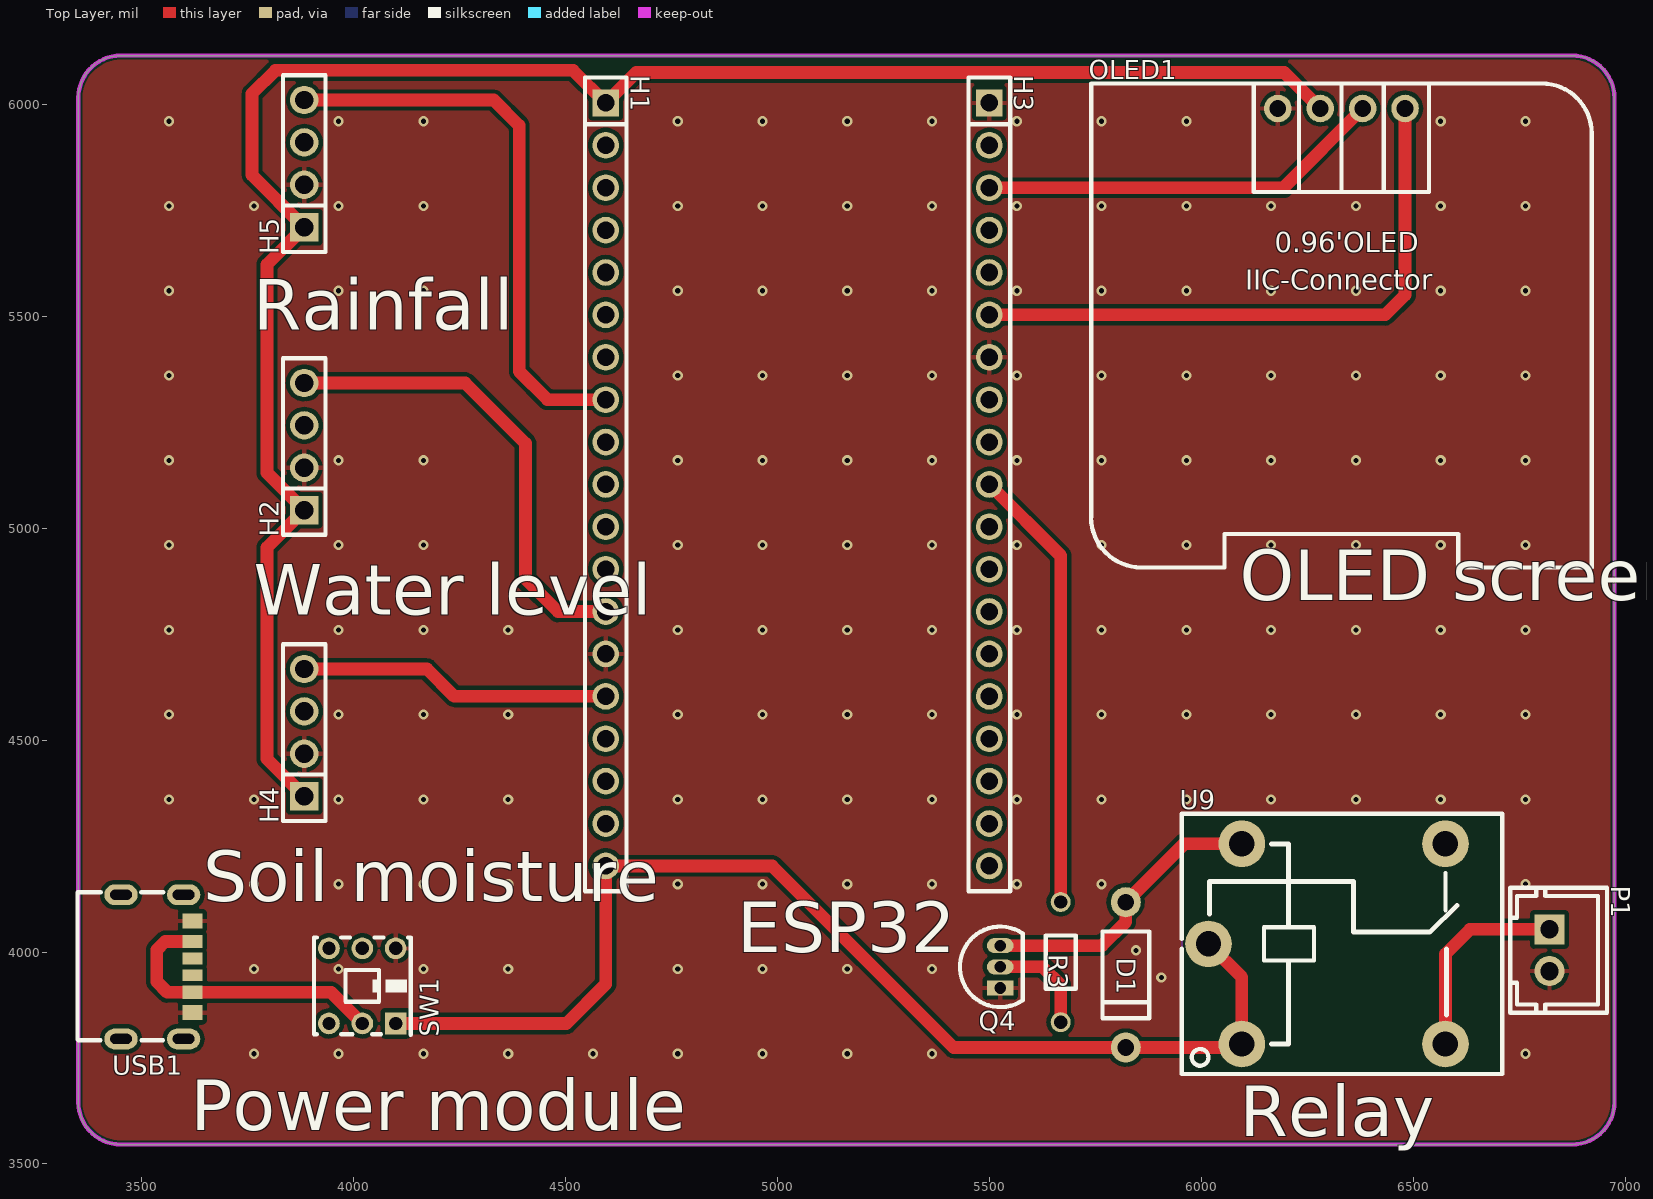
[diagram p0: Top Layer view]
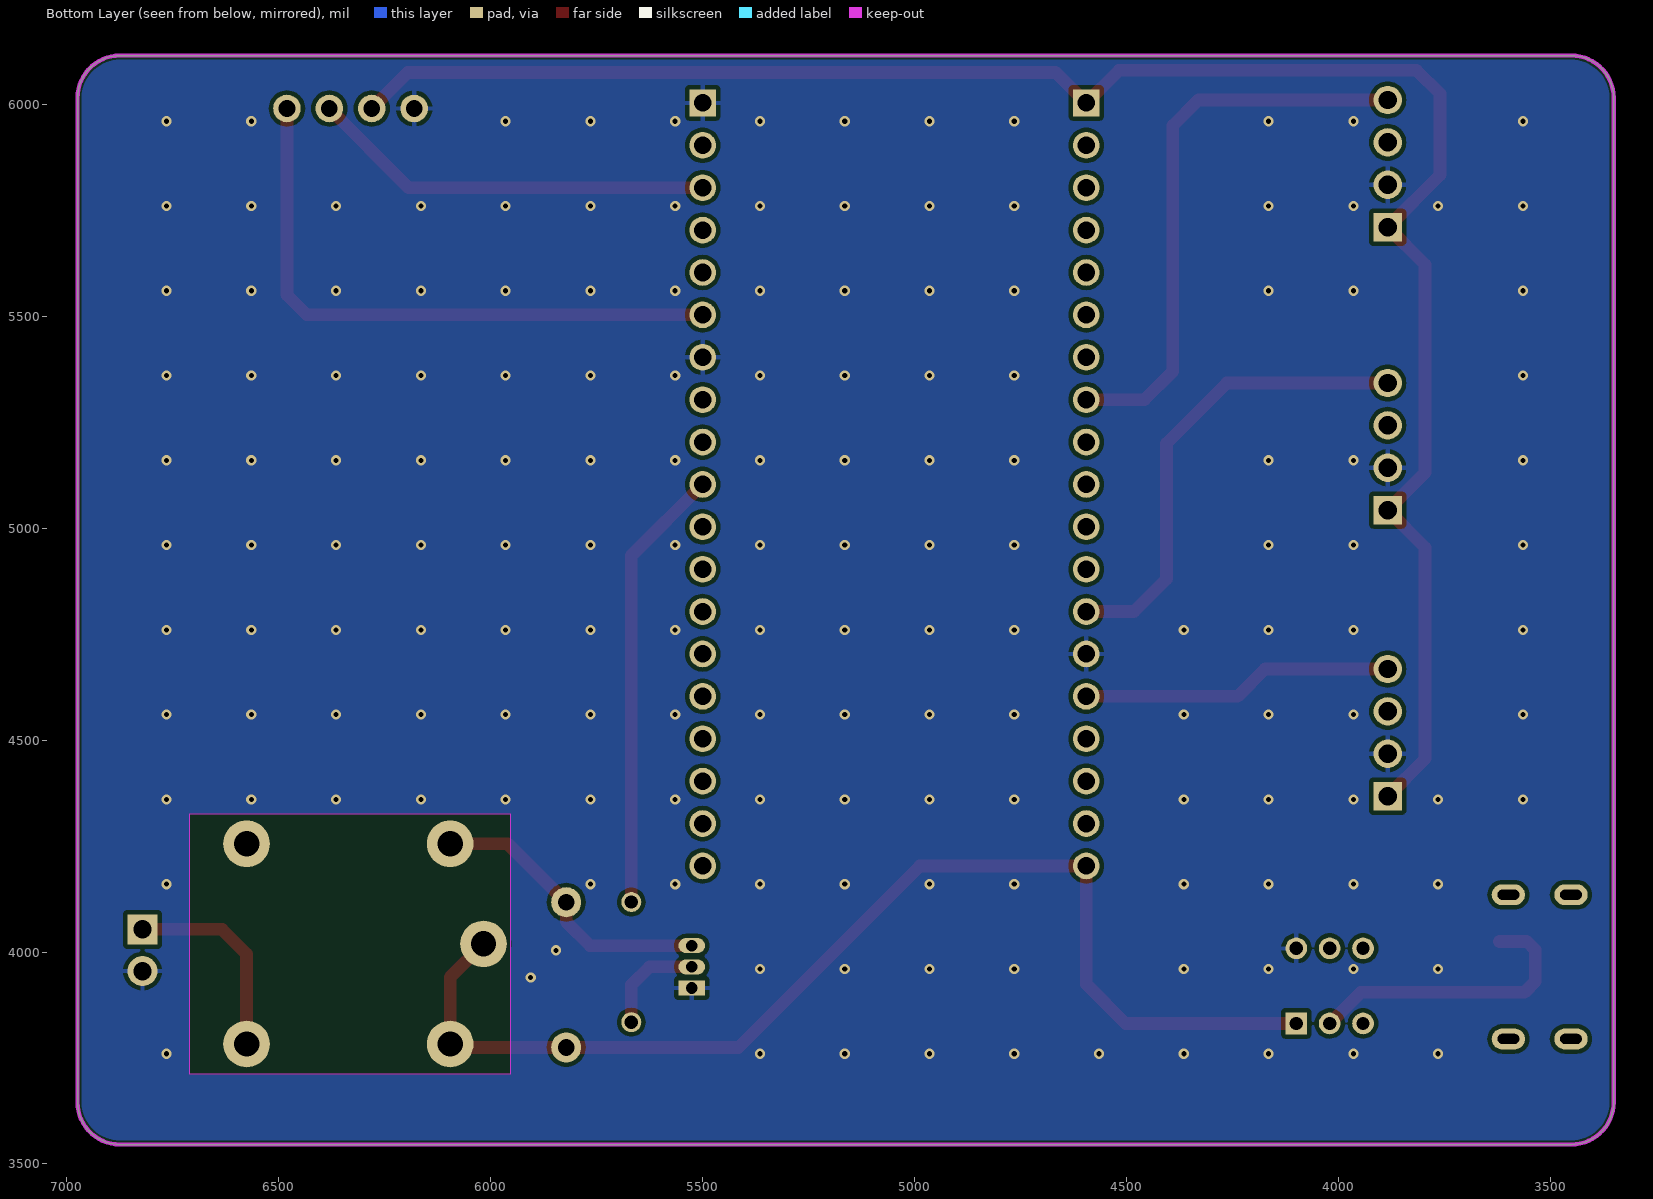
[diagram p1: Bottom Layer view, seen from below]
# Altium PCB MISC89058.pcbdoc
Units mil, origin at the board's own origin, x right, y up, seen from the top; angles counter-clockwise.
Board outline 3624.13 x 2569.13 mil, 2 copper layers (Top Layer, Bottom Layer), stack 62.206 mil thick; 13 components, 40 nets, 84 pads, 158 vias.

## Layer stack, top to bottom
Top Solder Mask Layer: solder mask 0.394, Dk 3.3
Top Layer: signal copper 1.379
Dielectric1: surface 59.449, FR4, Dk 4.5
Bottom Layer: signal copper 1.378
Bottom Solder Mask Layer: solder mask 0.394, Dk 3.3

## Board outline
3450,6115 ccw(c3450,6015) 3350,6015 3350,3645.87 ccw(c3450,3645.87) 3450,3545.87 6874.13,3545.87 ccw(c6874.13,3645.87) 6974.13,3645.87 6974.13,6015 ccw(c6874.13,6015) 6874.13,6115

## Design rules (kind name [scope] priority, off if disabled: settings)
BoardOutlineClearance copperThickness2oz_1 [All] p2 off: genericclearance=7.99 ignorepadtopadclearanceinfootprint=FALSE except(0: Arc-SplitContinuation Track-SplitContinuation SMDPad-SplitContinuation THPad-SplitContinuation Via-SplitContinuation Fill-SplitContinuation Region-SplitContinuation Poly-SplitContinuation Text-SplitContinuation Hole-SplitContinuation; 5.98: Arc-CutoutEdge Track-CutoutEdge SMDPad-CutoutEdge THPad-CutoutEdge Via-CutoutEdge Text-CutoutEdge; 6.9: Hole-OutlineEdge Hole-CutoutEdge; 10: Poly-OutlineEdge Poly-CutoutEdge; 11.81: Arc-OutlineEdge Track-OutlineEdge SMDPad-OutlineEdge THPad-OutlineEdge Via-OutlineEdge Fill-OutlineEdge Region-OutlineEdge Text-OutlineEdge Fill-CutoutEdge Region-CutoutEdge)
BoardOutlineClearance Plane_innerPlane_1 [All] p4 off: genericclearance=4.02 ignorepadtopadclearanceinfootprint=FALSE except(0: Arc-SplitContinuation Track-SplitContinuation SMDPad-SplitContinuation THPad-SplitContinuation Via-SplitContinuation Fill-SplitContinuation Region-SplitContinuation Poly-SplitContinuation Text-SplitContinuation Hole-SplitContinuation; 5.98: Arc-CutoutEdge Track-CutoutEdge SMDPad-CutoutEdge THPad-CutoutEdge Via-CutoutEdge Text-CutoutEdge; 6.9: Hole-OutlineEdge Hole-CutoutEdge; 10: Poly-OutlineEdge Poly-CutoutEdge; 11.81: Arc-OutlineEdge Track-OutlineEdge SMDPad-OutlineEdge THPad-OutlineEdge Via-OutlineEdge Fill-OutlineEdge Region-OutlineEdge Text-OutlineEdge Fill-CutoutEdge Region-CutoutEdge)
BoardOutlineClearance Copper_copperRegion_1 [All] p6 off: genericclearance=4.02 ignorepadtopadclearanceinfootprint=FALSE except(0: Arc-SplitContinuation Track-SplitContinuation SMDPad-SplitContinuation THPad-SplitContinuation Via-SplitContinuation Fill-SplitContinuation Region-SplitContinuation Poly-SplitContinuation Text-SplitContinuation Hole-SplitContinuation; 5.98: Arc-CutoutEdge Track-CutoutEdge SMDPad-CutoutEdge THPad-CutoutEdge Via-CutoutEdge Text-CutoutEdge; 6.9: Hole-OutlineEdge Hole-CutoutEdge; 10: Poly-OutlineEdge Poly-CutoutEdge; 11.81: Arc-OutlineEdge Track-OutlineEdge SMDPad-OutlineEdge THPad-OutlineEdge Via-OutlineEdge Fill-OutlineEdge Region-OutlineEdge Text-OutlineEdge Fill-CutoutEdge Region-CutoutEdge)
BoardOutlineClearance copperThickness1oz_1 [All] p8: genericclearance=4.02 ignorepadtopadclearanceinfootprint=FALSE except(0: Arc-SplitContinuation Track-SplitContinuation SMDPad-SplitContinuation THPad-SplitContinuation Via-SplitContinuation Fill-SplitContinuation Region-SplitContinuation Poly-SplitContinuation Text-SplitContinuation Hole-SplitContinuation; 5.98: Arc-CutoutEdge Track-CutoutEdge SMDPad-CutoutEdge THPad-CutoutEdge Via-CutoutEdge Text-CutoutEdge; 6.9: Hole-OutlineEdge Hole-CutoutEdge; 10: Poly-OutlineEdge Poly-CutoutEdge; 11.81: Arc-OutlineEdge Track-OutlineEdge SMDPad-OutlineEdge THPad-OutlineEdge Via-OutlineEdge Fill-OutlineEdge Region-OutlineEdge Text-OutlineEdge Fill-CutoutEdge Region-CutoutEdge)
Clearance copperThickness2oz [All] p1 off: gap=7.99 ignorepadtopadclearanceinfootprint=FALSE except(5.98: SMDPad-Track SMDPad-SMDPad THPad-Track SMDPad-THPad THPad-THPad Track-Via SMDPad-Via THPad-Via Via-Via Fill-SMDPad Region-SMDPad Fill-THPad Region-THPad Fill-Via Region-Via Fill-Fill Fill-Region Region-Region Arc-Track Arc-SMDPad Arc-THPad Arc-Via Fill-Arc Region-Arc Arc-Arc Text-Track SMDPad-Text Text-THPad Text-Via Fill-Text Region-Text Arc-Text Text-Text; 6.9: Hole-Track Hole-SMDPad Hole-THPad Hole-Via Fill-Hole Region-Hole Hole-Arc Hole-Text; 10: Poly-Track Poly-SMDPad Poly-THPad Poly-Via Poly-Fill Poly-Region Poly-Poly Poly-Arc Poly-Text Poly-Hole; 11.81: Fill-Track Region-Track)
Clearance Plane_innerPlane [All] p3 off: gap=4.02 ignorepadtopadclearanceinfootprint=FALSE except(5.98: SMDPad-Track SMDPad-SMDPad THPad-Track SMDPad-THPad THPad-THPad Track-Via SMDPad-Via THPad-Via Via-Via Fill-SMDPad Region-SMDPad Fill-THPad Region-THPad Fill-Via Region-Via Fill-Fill Fill-Region Region-Region Arc-Track Arc-SMDPad Arc-THPad Arc-Via Fill-Arc Region-Arc Arc-Arc Text-Track SMDPad-Text Text-THPad Text-Via Fill-Text Region-Text Arc-Text Text-Text; 6.9: Hole-Track Hole-SMDPad Hole-THPad Hole-Via Fill-Hole Region-Hole Hole-Arc Hole-Text; 10: Poly-Track Poly-SMDPad Poly-THPad Poly-Via Poly-Fill Poly-Region Poly-Poly Poly-Arc Poly-Text Poly-Hole; 11.81: Fill-Track Region-Track)
Clearance Copper_copperRegion [All] p5 off: gap=4.02 ignorepadtopadclearanceinfootprint=FALSE except(5.98: SMDPad-Track SMDPad-SMDPad THPad-Track SMDPad-THPad THPad-THPad Track-Via SMDPad-Via THPad-Via Via-Via Fill-SMDPad Region-SMDPad Fill-THPad Region-THPad Fill-Via Region-Via Fill-Fill Fill-Region Region-Region Arc-Track Arc-SMDPad Arc-THPad Arc-Via Fill-Arc Region-Arc Arc-Arc Text-Track SMDPad-Text Text-THPad Text-Via Fill-Text Region-Text Arc-Text Text-Text; 6.9: Hole-Track Hole-SMDPad Hole-THPad Hole-Via Fill-Hole Region-Hole Hole-Arc Hole-Text; 10: Poly-Track Poly-SMDPad Poly-THPad Poly-Via Poly-Fill Poly-Region Poly-Poly Poly-Arc Poly-Text Poly-Hole; 11.81: Fill-Track Region-Track)
Clearance copperThickness1oz [All] p7: gap=4.02 ignorepadtopadclearanceinfootprint=FALSE except(5.98: SMDPad-Track SMDPad-SMDPad THPad-Track SMDPad-THPad THPad-THPad Track-Via SMDPad-Via THPad-Via Via-Via Fill-SMDPad Region-SMDPad Fill-THPad Region-THPad Fill-Via Region-Via Fill-Fill Fill-Region Region-Region Arc-Track Arc-SMDPad Arc-THPad Arc-Via Fill-Arc Region-Arc Arc-Arc Text-Track SMDPad-Text Text-THPad Text-Via Fill-Text Region-Text Arc-Text Text-Text; 6.9: Hole-Track Hole-SMDPad Hole-THPad Hole-Via Fill-Hole Region-Hole Hole-Arc Hole-Text; 10: Poly-Track Poly-SMDPad Poly-THPad Poly-Via Poly-Fill Poly-Region Poly-Poly Poly-Arc Poly-Text Poly-Hole; 11.81: Fill-Track Region-Track)
DiffPairsRouting differentialPair [All] p1: maxlimit=6 minlimit=6 mostfreqgap=6 toplayer_minwidth=5 toplayer_prefwidth=10 toplayer_maxwidth=100 toplayer_mingap=6 toplayer_prefgap=6 toplayer_maxgap=6 bottomlayer_minwidth=5 bottomlayer_prefwidth=10 bottomlayer_maxwidth=100 bottomlayer_mingap=6 bottomlayer_prefgap=6 bottomlayer_maxgap=6 maxuncoupledlength=10
HoleToHoleClearance otherClearance [All] p1: gap=11.81 allowstackedmicrovias=TRUE
Length netLength [All] p1: minlimit=0 maxlimit=0
PasteMaskExpansion pasteMaskExpansion [All] p1: expansion=0
PlaneConnect innerPlane [All] p1: planeconnectstyle=Relief reliefexpansion=20 reliefentries=4 reliefconductorwidth=10 reliefairgap=10
PolygonConnect copperRegion [All] p1: connectstyle=Relief reliefconductorwidth=10 reliefentries=4 polygonreliefangle="90 Angle" airgapwidth=10 via.connectstyle=Relief via.reliefconductorwidth=10 via.reliefentries=4 via.polygonreliefangle="90 Angle" via.airgapwidth=10
RoutingVias viaSize [All] p1: holewidth=12.01 width=24.02 viastyle="Through Hole" minholewidth=11.81 minwidth=19.68 maxholewidth=248.03 maxwidth=393.7
SolderMaskExpansion solderMaskExpansion [IsVia] p1: expansion=-1000 istentingtop=TRUE
SolderMaskExpansion solderMaskExpansion [All] p2: expansion=2 istentingtop=FALSE
Width copperThickness2oz_2 [All] p1 off: maxlimit=100 minlimit=8 preferedwidth=10
Width copperThickness1oz_2 [All] p2: maxlimit=100 minlimit=5 preferedwidth=10

## Components (designator, comment, footprint, x,y, rotation, side; value= is the part's Value field where it differs from the comment)
D1 "" DO_1N4007 5821.22,3946.17 r90 top
H1 "C2897382" HDR-TH_19P-P2.54-V-F 4594.32,5103.13 r270 top
H2 "" HDR-TH_4P-P2.54-V-F 3883.17,5192.44 r90 top
H3 "C2897382" HDR-TH_19P-P2.54-V-F 5499.32,5103.13 r270 top
H4 "" HDR-TH_4P-P2.54-V-F 3883.17,4517.6 r90 top
H5 "" HDR-TH_4P-P2.54-V-F 3883.17,5860 r90 top
OLED1 "" 0.96OLED_4P 6330,5990 r0 top
P1 "WAFER-XH254Z-2A" CONN-TH_2P-P2.50_XH-2A_3045048 6820.83,4004.17 r270 top
Q4 "" S8050_TO_92 5525,3965 r90 top
R3 "1K" Res_1/8W 5665.22,3976.17 r270 top
SW1 "5.8 WSPT" SW-TH_6P-L5.8-W5.8-P2.00-LS4.5-TL_K8-5851E-L1 4020,3920 r180 top
U9 "SRD-12VDC-SL-C" RELAY-TH_SRD-XXVDC-XL-C 6295.83,4019.17 r0 top
USB1 "" "USB_ TYPE-C-6P" 3535,3970 r270 top

## Footprints (in the part's own frame and the unit in brackets; to place one, negate y for a bottom-side part, rotate by r counter-clockwise, add the part's x,y. Pads: shape width x height; smd on the part's side, far side on the other; paste and mask are expansions set on the pad)
0.96OLED_4P [mm]
  round 1.65 hole 1 copper offset 0,0: 1(-3.81,-0.001) 2(-1.27,0.002) 3(1.27,0.002) 4(3.81,0.002)
  silkscreen extent -15,-27.5 15,1.5
CONN-TH_2P-P2.50_XH-2A_3045048 [mm]
  rect 1.8x1.8 hole 1.1 paste+0 mask+0.05: 1(-1.25,0)
  round 1.8 hole 1.1 paste+0 mask+0.05: 2(1.25,0)
  silkscreen extent -3.75,-2.35 3.75,3.45
DO_1N4007 [mm]
  round 1.8 hole 1 paste+0 mask+0.051: 1(-4.35,0) 2(4.35,0)
  silkscreen extent -2.6,-1.4 2.6,1.4
HDR-TH_4P-P2.54-V-F [mm]
  rect 1.7x1.7 hole 1.1: 1(-3.81,0)
  round 1.7 hole 1.1: 2(-1.27,0) 3(1.27,0) 4(3.81,0)
  silkscreen extent -5.29,-1.27 5.29,1.27
HDR-TH_19P-P2.54-V-F [mm]
  rect 1.6x1.6 hole 1.05: 1(-22.86,0)
  round 1.6 hole 1.05: 2(-20.32,0) 3(-17.78,0) 4(-15.24,0) 5(-12.7,0) 6(-10.16,0) 7(-7.62,0) 8(-5.08,0) 9(-2.54,0) 10(0,0) 11(2.54,0) 12(5.08,0) 13(7.62,0) 14(10.16,0) 15(12.7,0) 16(15.24,0) 17(17.78,0) 18(20.32,0) 19(22.86,0)
  silkscreen extent -24.38,-1.25 24.38,1.25
RELAY-TH_SRD-XXVDC-XL-C [mil]
  round 110 hole 60: 1(-200.79,-236.22) 2(279.53,-236.2) 3(279.53,236.2) 4(-200.79,236.22) 5(-279.53,0)
  silkscreen extent -342,-307 413,307
Res_1/8W [mil]
  round 47.2 hole 31.5 paste+0 mask+2: 1(-141.7,2.48) 2(141.7,2.48)
  silkscreen extent -63,-33 63,38
S8050_TO_92 [mil]
  rect 35.4x63 hole 27.6 paste+0 mask+2: 1(-50,0)
  oval 35.4x63 hole 27.6 paste+0 mask+2: 2(0,0) 3(50,0)
  silkscreen extent -95,-53 95,95
SW-TH_6P-L5.8-W5.8-P2.00-LS4.5-TL_K8-5851E-L1 [mm]
  rect 1.3x1.3 hole 0.8 paste+0 mask+0.05: 1(-2,2.25)
  round 1.3 hole 0.8 paste+0 mask+0.05: 2(0,2.25) 3(2,2.25) 4(-2,-2.25) 5(0,-2.25) 6(2,-2.25)
  silkscreen extent -2.9,-2.9 2.9,2.92
"USB_ TYPE-C-6P" [mm]
  oval 1.25x2 hole 0.6 slot 1.3 at 90 deg paste+0 mask+0.05: 7(-4.193,1.611) 8(4.447,1.611) 9(-4.193,-2.139) 10(4.447,-2.139)
  rect 0.7x1.2 smd paste-100 mask+0.05: A5(-0.373,2.139) B5(0.627,2.139)
  rect 0.8x1.2 smd paste-100 mask+0.05: A9(1.647,2.139) B9(-1.393,2.139)
  rect 0.9x1.2 smd paste-100 mask+0.05: A12(2.877,2.139) B12(-2.623,2.139)
  silkscreen extent -4.34,-4.75 4.52,0.39

## Via types
v1: diameter 24.02, hole 12, Top Layer to Bottom Layer, 158 vias

## Nets (pads, with @x,y where several pads share a name; then routed paths per layer and width w, separated by ;. In a path a pad name is that pad's centre, name@x,y a point inside that pad or via, vN(x,y) a via of type N, cw(c..) or ccw(c..) an arc to the next point about the centre after c; other vN are vias at no path point)
$1N4284: SW1.2 USB1.A9 USB1.B9 | length 693.3
  Top Layer w30: USB1.B9 3554.84,4024.84 3535,4005 3535,3930 3559.84,3905.16 USB1.A9 3946.26,3905.16 SW1.2
$1N4728: P1.1 U9.2 | length 481.9
  Top Layer w30: U9.2 6575.36,3995.36 6633.38,4053.38 P1.1
$1N4736: D1.2 Q4.3 U9.4 | length 696.7
  Top Layer w30: Q4.3 5765,4015 5821.22,4071.22 D1.2 5959.17,4255.39 U9.4
$1N5006: Q4.2 R3.2 | length 248.2
  Top Layer w30: Q4.2 5625,3965 5667.7,3922.3 R3.2
+5V: D1.1 H1.19 SW1.1 U9.1 U9.5 | length 2763.1
  Top Layer w30: SW1.1 4501.42,3831.42 4594.32,3924.32 H1.19 4986.87,4203.13 5415.09,3774.91 D1.1 6087,3774.91 U9.1 6095.04,3940.43 U9.5
CLK: H3.19
CMD: H1.18
EN: H1.2
GND: H1.14 H2.2 H3.1 H3.7 H4.2 H5.2 OLED1.1 P1.2 Q4.1 SW1.4 USB1.A12 USB1.B12
  other v1: 3764.1,3759.97 3964.1,3759.97 4164.1,3759.97 4364.1,3759.97 4564.1,3759.97 4764.1,3759.97 4964.1,3759.97 5164.1,3759.97 5364.1,3759.97 6764.1,3759.97 5905,3940 3764.1,3959.97 3964.1,3959.97 4164.1,3959.97 4364.1,3959.97 4764.1,3959.97 4964.1,3959.97 5164.1,3959.97 5364.1,3959.97 5845.25,4004.01 3764.1,4159.97 3964.1,4159.97 4164.1,4159.97 4364.1,4159.97 4764.1,4159.97 4964.1,4159.97 5164.1,4159.97 5364.1,4159.97 5564.1,4159.97 5764.1,4159.97 6764.1,4159.97 3564.1,4359.97 3764.1,4359.97 3964.1,4359.97 4164.1,4359.97 4364.1,4359.97 4764.1,4359.97 4964.1,4359.97 5164.1,4359.97 5364.1,4359.97 5564.1,4359.97 5764.1,4359.97 5964.1,4359.97 6164.1,4359.97 6364.1,4359.97 6564.1,4359.97 6764.1,4359.97 3564.1,4559.97 3964.1,4559.97 4164.1,4559.97 4364.1,4559.97 4764.1,4559.97 4964.1,4559.97 5164.1,4559.97 5364.1,4559.97 5564.1,4559.97 5764.1,4559.97 5964.1,4559.97 6164.1,4559.97 6364.1,4559.97 6564.1,4559.97 6764.1,4559.97 3564.1,4759.97 3964.1,4759.97 4164.1,4759.97 4364.1,4759.97 4764.1,4759.97 4964.1,4759.97 5164.1,4759.97 5364.1,4759.97 5564.1,4759.97 5764.1,4759.97 5964.1,4759.97 6164.1,4759.97 6364.1,4759.97 6564.1,4759.97 6764.1,4759.97 3564.1,4959.97 3964.1,4959.97 4164.1,4959.97 4764.1,4959.97 4964.1,4959.97 5164.1,4959.97 5364.1,4959.97 5564.1,4959.97 5764.1,4959.97 5964.1,4959.97 6164.1,4959.97 6364.1,4959.97 6564.1,4959.97 6764.1,4959.97 3564.1,5159.97 3964.1,5159.97 4164.1,5159.97 4764.1,5159.97 4964.1,5159.97 5164.1,5159.97 5364.1,5159.97 5564.1,5159.97 5764.1,5159.97 5964.1,5159.97 6164.1,5159.97 6364.1,5159.97 6564.1,5159.97 6764.1,5159.97 3564.1,5359.97 4764.1,5359.97 4964.1,5359.97 5164.1,5359.97 5364.1,5359.97 5564.1,5359.97 5764.1,5359.97 5964.1,5359.97 6164.1,5359.97 6364.1,5359.97 6564.1,5359.97 6764.1,5359.97 3564.1,5559.97 3964.1,5559.97 4164.1,5559.97 4764.1,5559.97 4964.1,5559.97 5164.1,5559.97 5364.1,5559.97 5564.1,5559.97 5764.1,5559.97 5964.1,5559.97 6164.1,5559.97 6364.1,5559.97 6564.1,5559.97 6764.1,5559.97 3564.1,5759.97 3764.1,5759.97 3964.1,5759.97 4164.1,5759.97 4764.1,5759.97 4964.1,5759.97 5164.1,5759.97 5364.1,5759.97 5564.1,5759.97 5764.1,5759.97 5964.1,5759.97 6164.1,5759.97 6364.1,5759.97 6564.1,5759.97 6764.1,5759.97 3564.1,5959.97 3964.1,5959.97 4164.1,5959.97 4764.1,5959.97 4964.1,5959.97 5164.1,5959.97 5364.1,5959.97 5564.1,5959.97 5764.1,5959.97 5964.1,5959.97 6564.1,5959.97 6764.1,5959.97
P0: H3.14
P2: H3.15
P4: H3.13
P5: H3.10 R3.1 | length 1055
  Top Layer w30: H3.10 5667.7,4934.75 R3.1
P12: H1.13 H2.4 | length 1122
  Top Layer w30: H2.4 4262.56,5342.44 4405,5200 4405,4880 4481.87,4803.13 H1.13
P13: H1.15 H4.4 | length 737.9
  Top Layer w30: H4.4 4172.4,4667.6 4236.87,4603.13 H1.15
P14: H1.12
P15: H3.16
P16: H3.12
P17: H3.11
P18: H3.9
P19: H3.8
P21: H3.6 OLED1.4 | length 1440.1
  Top Layer w30: H3.6 6433.13,5503.13 6480,5550 OLED1.4@6480,5990.05
P22: H3.3 OLED1.3 | length 958.1
  Top Layer w30: H3.3 6193.08,5803.13 OLED1.3@6380,5990.05
P23: H3.2
P25: H1.9
P26: H1.10
P27: H1.11
P32: H1.7
P33: H1.8 H5.4 | length 1343.7
  Top Layer w30: H5.4 4330,6010 4390,5950 4390,5370 4456.87,5303.13 H1.8
P34: H1.5
P35: H1.6
RX0: H3.5
SD0: H3.18
SD1: H3.17
SD2: H1.16
SD3: H1.17
SVN: H1.4
SVP: H1.3
TX0: H3.4
VCC: H1.1 H2.1 H4.1 H5.1 OLED1.2 | length 4494.1
  Top Layer w30: H4.1 3795,4455.77 3795,4954.27 H2.1 3795,5130.6 3795,5621.83 H5.1 3760,5833.17 3760,6025 3815,6080 4517.44,6080 H1.1 4666.19,6075 6195.05,6075 OLED1.2@6280,5990.05
pads on no net: H2.3 H4.3 H5.3 SW1.3 SW1.5 SW1.6 U9.3 USB1.7 USB1.8 USB1.9 USB1.10 USB1.A5 USB1.B5

## Polygon pours and split planes (outlines as drawn)
GND on Top Layer (solid, remove dead copper, pour order 0): 3000,6980 3000,3000 7000,3000 7000,6980
GND on Bottom Layer (solid, remove dead copper, pour order 2): 3000,6985 3000,3010 6995,3010 6995,6985

## Keep-outs
Board Outline Layer:
  region: 5953.34,4326.26 5953.34,3712.08 6709.25,3712.08 6709.25,4326.26
  lines w10: 3350,3645.87 3350,6015 cw(c3450,6015) 3450,6115 6874.13,6115 cw(c6874.13,6015) 6974.13,6015 6974.13,3645.87 cw(c6874.13,3645.87) 6874.13,3545.87 3450,3545.87 cw(c3450,3645.87) 3350,3645.87

## Silkscreen, mask and mechanical layers (free items; w line width, h text height)
Top Silkscreen Layer:
  text "Rainfall" at 3762.99,5467.67 h120
  text "OLED screen" at 6090,4830 h120
  text "Water level" at 3763.74,4795.75 h120
  text "Soil moisture" at 3644.19,4120 h120
  text "ESP32" at 4905,4000 h120
  text "Power module" at 3615,3580 h120
  text "Relay" at 6090,3565 h120